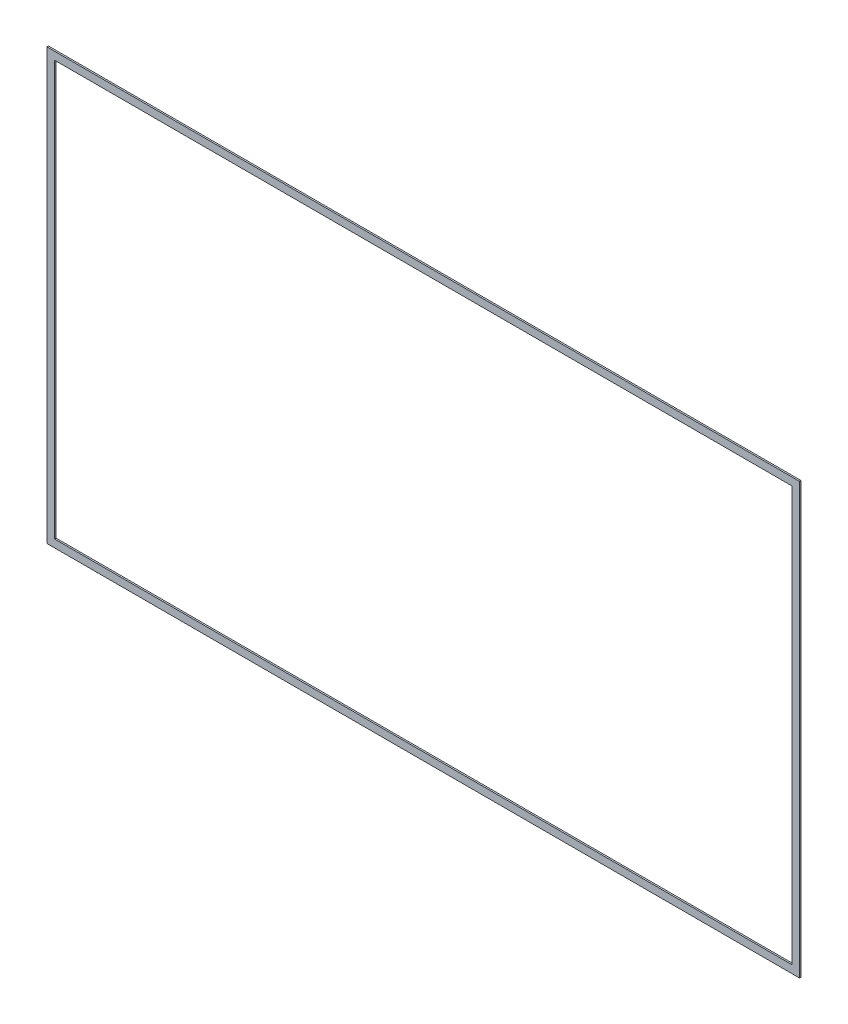
from build123d import *

# Parameters (mm, degrees)
SKETCH_1_W      = 974.6
SKETCH_1_H      = 557
SKETCH_1_W_2    = 954.6
SKETCH_1_H_2    = 537
EXTRUDE_1_DEPTH = 2
FILLET_1_R      = 0.2


with BuildPart() as part:
    # 草图1 → 凸台-拉伸1 (new body)
    with BuildSketch(Plane.XY):
        Rectangle(SKETCH_1_W, SKETCH_1_H)
        Rectangle(SKETCH_1_W_2, SKETCH_1_H_2, mode=Mode.SUBTRACT)
    extrude(amount=EXTRUDE_1_DEPTH)

    # 圆角1
    fillet_1_edges = [part.edges().sort_by_distance(p)[0] for p in [
        (477.3, -268.5, 1),
        (477.3, 268.5, 1),
        (-477.3, 268.5, 1),
        (-477.3, -268.5, 1),
    ]]
    fillet(fillet_1_edges, radius=FILLET_1_R)


solid = part.part
